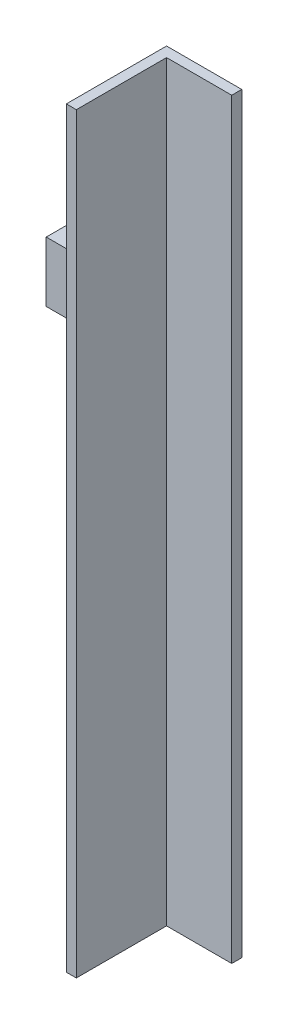
from build123d import *

# Parameters (mm, degrees)
SKETCH1_W           = 15
SKETCH1_H           = 70
BOSS_EXTRUDE1_DEPTH = 20
SKETCH2_W           = 13
SKETCH2_H           = 18
CUT_EXTRUDE1_DEPTH  = 154
BOSS_EXTRUDE2_DEPTH = 80
SKETCH4_W           = 12
SKETCH4_H           = 12
SKETCH4_R           = 3.5
BOSS_EXTRUDE4_DEPTH = 10


with BuildPart() as part:
    # Sketch1 → Boss-Extrude1 (new body)
    with BuildSketch(Plane.XY):
        with Locations((100, 0)):
            Rectangle(SKETCH1_W, SKETCH1_H)
    extrude(amount=BOSS_EXTRUDE1_DEPTH)

    # Sketch2 → Cut-Extrude1 (cut)
    with BuildSketch(Plane(origin=(0, -35, 0), x_dir=(-1, 0, 0), z_dir=(0, -1, 0))):
        with Locations((-101, -11)):
            Rectangle(SKETCH2_W, SKETCH2_H)
    extrude(amount=-CUT_EXTRUDE1_DEPTH, mode=Mode.SUBTRACT)

    # Sketch3 → Boss-Extrude2 (add)
    with BuildSketch(Plane.XZ.offset(35)):
        Polygon((107.5, 0), (107.5, 2), (94.5, 2), (94.5, 20), (92.5, 20), (92.5, 0), align=None)
    extrude(amount=BOSS_EXTRUDE2_DEPTH)

    # Sketch4 → Boss-Extrude4 (add)
    with BuildSketch(Plane(origin=(94.5, 0, 0), x_dir=(0, 0, -1), z_dir=(1, 0, 0))):
        with Locations((-10, 0)):
            Rectangle(SKETCH4_W, SKETCH4_H)
        with Locations(Location((-10, 0, 0), (0, 0, 90))):
            Circle(SKETCH4_R, mode=Mode.SUBTRACT)
    extrude(amount=-BOSS_EXTRUDE4_DEPTH)


solid = part.part
